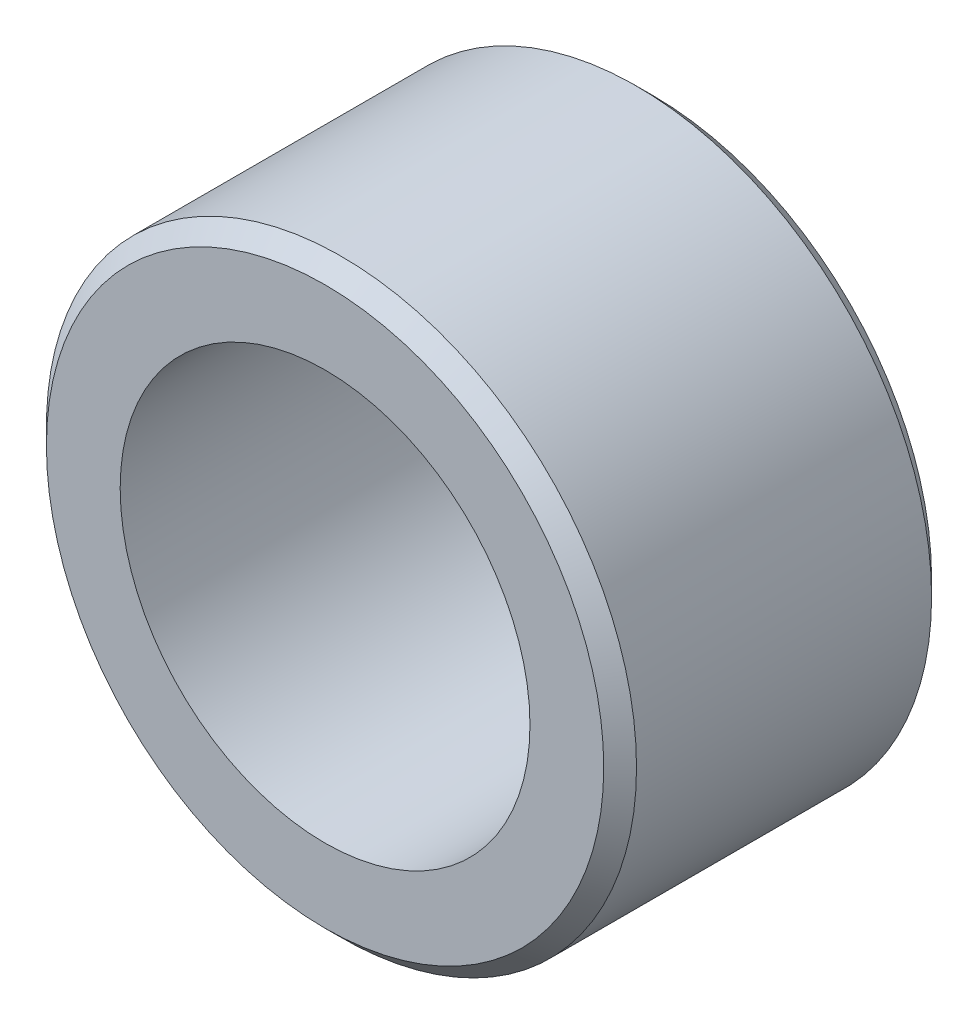
SolidWorks part; units mm, degrees
material "黄铜"
ref_plane "Front Plane" through (0, 0, 0) normal (0, 0, 1) x (1, 0, 0)
ref_plane "Top Plane" through (0, 0, 0) normal (0, 1, 0) x (1, 0, 0)
ref_plane "Right Plane" through (0, 0, 0) normal (1, 0, 0) x (0, 0, -1)
sketch "Sketch1" plane through (0, 0, 0) normal (0, 0, 1) x (1, 0, 0)
  circle A0 centre (0, 0) radius 9
  circle A1 centre (0, 0) radius 6.25
  dimension "D1" = 18
  dimension "D2" = 12.5
extrude "Boss-Extrude1" add sketch "Sketch1" along normal blind 10
chamfer "Chamfer1" distance 0.5 angle 45 2 edges at (9, 0, 10) (9, 0, 0)
